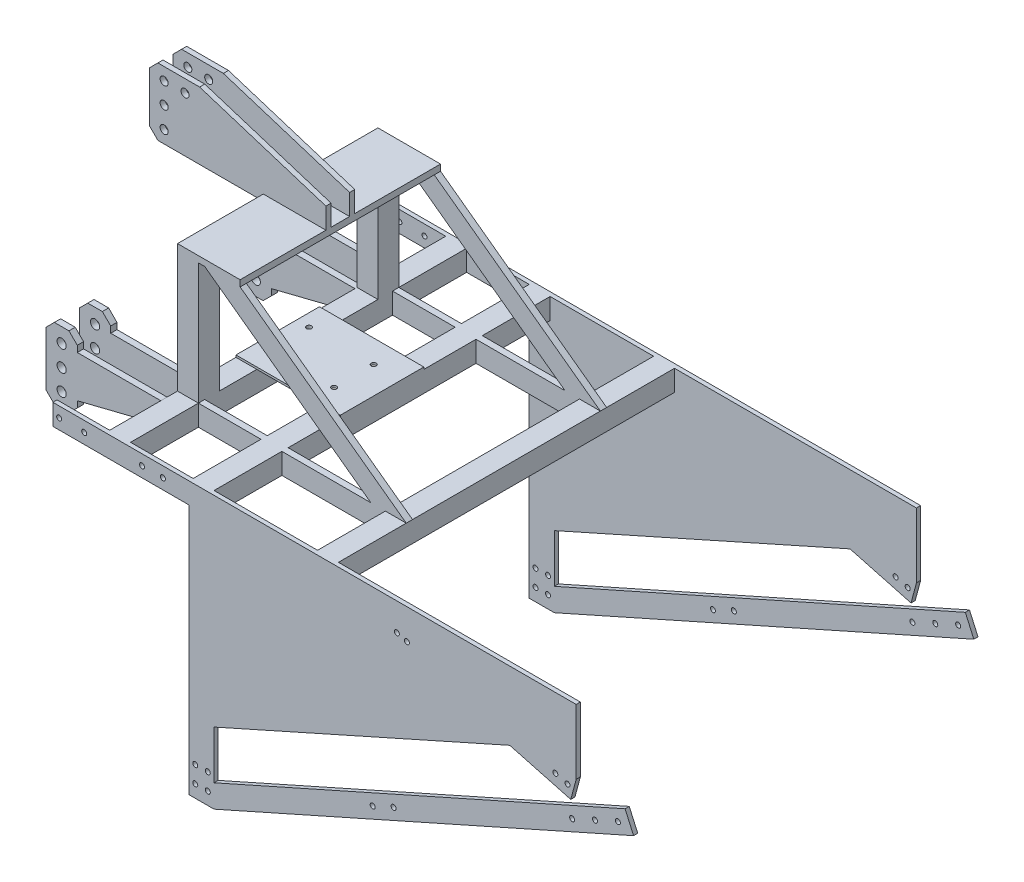
SolidWorks part; units mm, degrees
ref_plane "前视基准面" through (0, 0, 0) normal (0, 0, 1) x (1, 0, 0)
ref_plane "上视基准面" through (0, 0, 0) normal (0, 1, 0) x (1, 0, 0)
ref_plane "右视基准面" through (0, 0, 0) normal (1, 0, 0) x (0, 0, -1)
sketch "草图1" plane through (0, 0, 0) normal (0, 0, 1) x (1, 0, 0)
  line L1 (0, 0) -> (50, 0)
  line L2 (0, 0) -> (0, 50)
  line L3 (0, 50) -> (50, 50)
  line L4 (50, 0) -> (50, 50)
  line L5 (5, 5) -> (45, 5)
  line L6 (5, 5) -> (5, 45)
  line L7 (5, 45) -> (45, 45)
  line L8 (45, 5) -> (45, 45)
  dimension "D1" = 5
  dimension "D2" = 5
  dimension "D3" = 5
  dimension "D4" = 5
extrude "凸台-拉伸1" add sketch "草图1" along normal mid plane 805
sketch "草图2" plane through (0, 0, 402.5) normal (0, 0, 1) x (1, 0, 0)
  line L0 (-237.8943, -601) -> (767.0057, -153.5897)
  line L1 (50, 50) -> (-250, 50)
  line L2 (746.6689, -107.9124) -> (767.0057, -153.5897)
  line L3 (43.4174, 0) -> (-237.8943, 0)
  line L4 (629.5555, -105.2914) -> (616.6145, -153.5877)
  line L5 (-250, 50) -> (-297.8943, 50)
  line L6 (-237.8943, 0) -> (-237.8943, -546.2682)
  line L7 (-237.8943, -601) -> (-297.8943, -601)
  line L8 (-297.8943, 0) -> (-297.8943, -601)
  line L9 (-297.8943, 50) -> (-497.8943, 50)
  line L10 (50, 50) -> (629.5555, -105.2914)
  line L11 (43.4174, 0) -> (616.6145, -153.5877)
  line L12 (-497.8943, 50) -> (-577.8943, 50)
  line L13 (-497.8943, 0) -> (-297.8943, 0)
  line L15 (-577.8943, 0) -> (-497.8943, 0)
  line L16 (-385.3943, 150) -> (-385.3943, -14.3313) construction
  line L17 (-577.8943, 50) -> (-623.8943, 50)
  line L18 (-623.8943, 50) -> (-623.8943, 0)
  line L19 (746.6689, -107.9124) -> (-237.8943, -546.2682)
  line L20 (-623.8943, 0) -> (-577.8943, 0)
  circle A0 centre (-282.8943, -531) radius 6
  circle A1 centre (-252.8943, -531) radius 6
  circle A2 centre (-282.8943, -571) radius 6
  circle A3 centre (-252.8943, -571) radius 6
  circle A4 centre (142.1057, -404.4472) radius 6
  circle A5 centre (-267.8943, -248) radius 6
  circle A6 centre (-267.8943, -284) radius 6
  circle A7 centre (192.1057, -382.1858) radius 6
  circle A8 centre (729.4309, -142.9532) radius 6
  circle A9 centre (674.6182, -167.3574) radius 6
  circle A10 centre (619.8055, -191.7616) radius 6
  circle A11 centre (608.5961, -125.5573) radius 6
  circle A12 centre (579.6184, -117.7927) radius 6
  circle A13 centre (-608.8943, 25) radius 6
  circle A14 centre (-548.8943, 25) radius 6
  circle A15 centre (-360.3943, 25) radius 6
  circle A16 centre (-410.3943, 25) radius 6
  circle A17 centre (200, -16.0743) radius 6
  circle A18 centre (224.1481, -22.5448) radius 6
  dimension "D4" = 15
  dimension "D5" = 30
  dimension "D6" = 15
  dimension "D7" = 30
  dimension "D8" = 30
  dimension "D9" = 40
  dimension "D10" = 36
  dimension "D11" = 248
  dimension "D12" = 15
  dimension "D2" = 30
  dimension "D13" = 30
  dimension "D17" = 50
  dimension "D19" = 30
  dimension "D20" = 60
  dimension "D21" = 60
  dimension "D22" = 15
  dimension "D23" = 30
  dimension "D27" = 25
  dimension "D28" = 25
  dimension "D1" = 24
  dimension "D3" = 601
  dimension "D14" = 60
  dimension "D15" = 601
  dimension "D16" = 50
  dimension "D18" = 1100
  dimension "D25" = 200
extrude "凸台-拉伸2" add sketch "草图2" along normal blind 10
sketch "草图3" plane through (0, 0, 402.5) normal (0, 0, -1) x (-1, 0, 0)
  line L1 (297.8943, 50) -> (247.8943, 50)
  line L2 (297.8943, 50) -> (297.8943, 0)
  line L3 (297.8943, 0) -> (247.8943, 0)
  line L4 (247.8943, 50) -> (247.8943, 0)
  line L5 (252.8943, 5) -> (292.8943, 5)
  line L6 (252.8943, 5) -> (252.8943, 45)
  line L7 (252.8943, 45) -> (292.8943, 45)
  line L8 (292.8943, 5) -> (292.8943, 45)
  dimension "D1" = 40
  dimension "D2" = 5
  dimension "D3" = 5
extrude "凸台-拉伸3" add sketch "草图3" along normal up to surface (805 mm away) up to face at (25, 25, -402.5)
sketch "草图4" plane through (0, 0, -402.5) normal (0, 0, -1) x (-1, 0, 0)
  line L0 (-612.8098, -100.8044) -> (-50, 50)
  line L1 (-50, 50) -> (297.8943, 50)
  line L2 (297.8943, 0) -> (297.8943, -601)
  line L3 (297.8943, -601) -> (237.8943, -601)
  line L4 (237.8943, -601) -> (-767.0057, -153.5897)
  line L5 (297.8943, 0) -> (497.8943, 0)
  line L6 (-746.6689, -107.9124) -> (237.8943, -546.2682)
  line L7 (237.8943, -546.2682) -> (237.8943, 0)
  line L8 (237.8943, 0) -> (-43.4174, 0)
  line L9 (-767.0057, -153.5897) -> (-746.6689, -107.9124)
  line L10 (497.8943, 50) -> (577.8943, 50)
  line L11 (-43.4174, 0) -> (-616.6145, -153.5877)
  line L12 (-616.6145, -153.5877) -> (-629.5555, -105.2914)
  line L13 (-629.5555, -105.2914) -> (-612.8098, -100.8044)
  line L14 (497.8943, 50) -> (297.8943, 50)
  line L15 (-50, 50) -> (623.8943, 50) construction
  line L17 (577.8943, 0) -> (497.8943, 0)
  line L18 (577.8943, 50) -> (623.8943, 50)
  line L19 (623.8943, 50) -> (623.8943, 0)
  line L20 (623.8943, 50) -> (623.8943, 0) construction
  line L21 (623.8943, 0) -> (577.8943, 0)
  circle A0 centre (267.8943, -248) radius 6
  circle A1 centre (267.8943, -284) radius 6
  circle A2 centre (252.8943, -531) radius 6
  circle A3 centre (282.8943, -531) radius 6
  circle A4 centre (282.8943, -571) radius 6
  circle A5 centre (252.8943, -571) radius 6
  circle A6 centre (-192.1057, -382.1858) radius 6
  circle A7 centre (-142.1057, -404.4472) radius 6
  circle A8 centre (-608.5961, -125.5573) radius 6
  circle A9 centre (-579.6184, -117.7927) radius 6
  circle A10 centre (-674.6182, -167.3574) radius 6
  circle A11 centre (-729.4309, -142.9532) radius 6
  circle A12 centre (-619.8055, -191.7616) radius 6
  circle A13 centre (608.8943, 25) radius 6
  circle A14 centre (548.8943, 25) radius 6
extrude "凸台-拉伸4" add sketch "草图4" along normal blind 10
ref_plane "基准面1" through (0, 0, 232.5) normal (0, 0, 1) x (1, 0, 0)
ref_plane "基准面2" through (0, 0, -232.5) normal (0, 0, 1) x (1, 0, 0)
sketch "草图5" plane through (0, 0, 232.5) normal (0, 0, 1) x (1, 0, 0)
  line L0 (-497.8943, 50) -> (-497.8943, 0)
  line L1 (-497.8943, 50) -> (-697.8943, 50)
  line L2 (-697.8943, 50) -> (-697.8943, 65)
  line L3 (-717.8943, 85) -> (-752.8943, 85)
  line L4 (-772.8943, 65) -> (-772.8943, -65)
  line L5 (-752.8943, -85) -> (-717.8943, -85)
  line L6 (-752.8943, 85) -> (-772.8943, 65)
  line L7 (-297.8943, 0) -> (-297.8943, -601) construction
  line L8 (-697.8943, -65) -> (-697.8943, -50)
  line L9 (-697.8943, 65) -> (-717.8943, 85)
  line L10 (-697.8943, -50) -> (-497.8943, 0)
  line L11 (-717.8943, -85) -> (-697.8943, -65)
  line L12 (-772.8943, -65) -> (-752.8943, -85)
  circle A2 centre (-735.3943, 50) radius 11
  circle A3 centre (-735.3943, 0) radius 11
  circle A5 centre (-735.3943, -50) radius 11
  point P0 (-772.8943, -85)
  point P1 (-697.8943, 85)
  point P6 (-772.8943, 85)
  point P12 (-697.8943, -85)
  dimension "D7" = 50
  dimension "D2" = 35
  dimension "D4" = 75
  dimension "D6" = 35
  dimension "D9" = 200
extrude "凸台-拉伸5" add sketch "草图5" along normal mid plane 95
sketch "草图7" plane through (0, 0, -232.5) normal (0, 0, 1) x (1, 0, 0)
  line L0 (-772.8943, 65) -> (-772.8943, -65)
  line L1 (-752.8943, -85) -> (-717.8943, -85)
  line L2 (-697.8943, -65) -> (-697.8943, -50)
  line L4 (-497.8943, 0) -> (-497.8943, 50)
  line L5 (-497.8943, 50) -> (-697.8943, 50)
  line L6 (-697.8943, 50) -> (-697.8943, 65)
  line L7 (-717.8943, 85) -> (-752.8943, 85)
  line L8 (-697.8943, 65) -> (-717.8943, 85)
  line L9 (-752.8943, 85) -> (-772.8943, 65)
  line L10 (-772.8943, -65) -> (-752.8943, -85)
  line L11 (-697.8943, -50) -> (-497.8943, 0)
  line L12 (-717.8943, -85) -> (-697.8943, -65)
  circle A2 centre (-735.3943, 50) radius 11
  circle A3 centre (-735.3943, 0) radius 11
  circle A5 centre (-735.3943, -50) radius 11
  point P0 (-772.8943, 85)
  point P1 (-772.8943, -85)
  point P3 (-697.8943, -85)
  point P12 (-697.8943, 85)
  point P22 (-772.8943, 85)
  dimension "D1" = 50
extrude "凸台-拉伸6" add sketch "草图7" along normal mid plane 95 separate body
sketch "草图10" plane through (0, 85, 0) normal (0, 1, 0) x (1, 0, 0)
  line L0 (-497.8943, 280) -> (-697.8943, 280) construction
  line L1 (-804.976, 265) -> (-454.4331, 265)
  line L2 (-804.976, 265) -> (-804.976, 200)
  line L3 (-804.976, 200) -> (-454.4331, 200)
  line L4 (-454.4331, 265) -> (-454.4331, 200)
  dimension "D1" = 65
  dimension "D2" = 15
extrude "切除-拉伸6" cut sketch "草图10" against normal through all
sketch "草图11" plane through (0, 0, -402.5) normal (0, 0, 1) x (1, 0, 0)
  line L1 (-497.8943, 50) -> (-447.8943, 50)
  line L2 (-497.8943, 50) -> (-497.8943, 0)
  line L3 (-497.8943, 0) -> (-447.8943, 0)
  line L4 (-447.8943, 50) -> (-447.8943, 0)
  line L5 (-492.8943, 45.3872) -> (-452.8943, 45.3872)
  line L6 (-492.8943, 45.3872) -> (-492.8943, 5.3872)
  line L7 (-492.8943, 5.3872) -> (-452.8943, 5.3872)
  line L8 (-452.8943, 45.3872) -> (-452.8943, 5.3872)
  dimension "D1" = 40
  dimension "D2" = 50
  dimension "D3" = 5
extrude "凸台-拉伸7" add sketch "草图11" along normal up to surface (805 mm away) up to face at (198.1057, -382.1858, 402.5)
sketch "草图12" plane through (0, 85, 0) normal (0, 1, 0) x (1, 0, 0)
  line L0 (-497.8943, -402.5) -> (-497.8943, 185) construction
  line L1 (-813.5215, -200) -> (-497.8943, -200)
  line L2 (-813.5215, -200) -> (-813.5215, -265)
  line L3 (-813.5215, -265) -> (-497.8943, -265)
  line L4 (-497.8943, -200) -> (-497.8943, -265)
  line L6 (-497.8943, -280) -> (-697.8943, -280) construction
  dimension "D1" = 65
  dimension "D2" = 15
extrude "切除-拉伸7" cut sketch "草图12" against normal through all
sketch "草图13" plane through (0, 0, 232.5) normal (0, 0, 1) x (1, 0, 0)
  line L1 (-447.8943, 50) -> (0, 50)
  line L2 (-447.8943, 50) -> (-447.8943, 0)
  line L3 (-447.8943, 0) -> (0, 0)
  line L4 (0, 50) -> (0, 0)
extrude "凸台-拉伸8" add sketch "草图13" along normal mid plane 15
sketch "草图14" plane through (0, 0, -232.5) normal (0, 0, 1) x (1, 0, 0)
  line L1 (-447.8943, 50) -> (0, 50)
  line L2 (-447.8943, 50) -> (-447.8943, 0)
  line L3 (-447.8943, 0) -> (0, 0)
  line L4 (0, 50) -> (0, 0)
extrude "凸台-拉伸9" add sketch "草图14" along normal mid plane 15
sketch "草图15" plane through (0, 0, 0) normal (0, 0, 1) x (1, 0, 0)
  line L0 (-670.3943, 341) -> (-297.8943, 341)
  line L1 (-770.3943, 481.7) -> (-750.3943, 501.7)
  line L3 (-770.3943, 361) -> (-750.3943, 341)
  line L6 (-297.8943, 341) -> (-297.8943, 404.9245)
  line L7 (-750.3943, 501.7) -> (-645.3943, 501.7)
  line L8 (-297.8943, 404.9245) -> (-645.3943, 501.7)
  line L9 (-770.3943, 371) -> (-770.3943, 361)
  line L10 (-750.3943, 341) -> (-670.3943, 341)
  line L11 (-770.3943, 371) -> (-770.3943, 481.7)
  circle A0 centre (-735.3943, 471.7) radius 9.65
  circle A3 centre (-735.3943, 371) radius 9.65
  circle A4 centre (-735.3943, 421.7) radius 9.65
  circle A6 centre (-685.3943, 471.7) radius 9.65
  point P20 (-770.3943, 341)
  dimension "D1" = 19.3
  dimension "D2" = 50
  dimension "D5" = 50
extrude "凸台-拉伸10" add sketch "草图15" along normal mid plane 69 separate body
sketch "草图16" plane through (0, 501.7, 0) normal (0, 1, 0) x (1, 0, 0)
  line L0 (-645.3943, 34.5) -> (-750.3943, 34.5) construction
  line L1 (-821.6581, 22.25) -> (-221.0953, 22.25)
  line L2 (-821.6581, 22.25) -> (-821.6581, -22.25)
  line L3 (-821.6581, -22.25) -> (-221.0953, -22.25)
  line L4 (-221.0953, 22.25) -> (-221.0953, -22.25)
  dimension "D1" = 44.5
  dimension "D2" = 600.5628
  dimension "D3" = 12.25
extrude "切除-拉伸8" cut sketch "草图16" against normal blind 200
sketch "草图19" plane through (-497.8943, 0, 0) normal (-1, 0, 0) x (0, 0, 1)
  line L0 (-240, 341) -> (-240, 356)
  line L1 (-240, 356) -> (240, 356)
  line L2 (-240, 341) -> (240, 341)
  line L3 (240, 356) -> (240, 341)
extrude "凸台-拉伸11" add sketch "草图19" against normal blind 200
sketch "草图20" plane through (0, 0, 240) normal (0, 0, 1) x (1, 0, 0)
  line L0 (-347.8943, 341) -> (50, 50)
  line L5 (-34.6995, 50) -> (-432.5938, 341)
  line L6 (-347.8943, 341) -> (-432.5938, 341)
  line L7 (50, 50) -> (-34.6995, 50)
  line L9 (-297.8943, 341) -> (-497.8943, 341) construction
  line L12 (50, 50) -> (-623.8943, 50) construction
extrude "凸台-拉伸12" add sketch "草图20" against normal blind 15
sketch "草图21" plane through (0, 0, -225) normal (0, 0, 1) x (1, 0, 0)
  line L0 (50, 50) -> (-347.8943, 341)
  line L1 (-347.8943, 341) -> (-432.5938, 341)
  line L2 (-432.5938, 341) -> (-34.6995, 50)
  line L3 (-34.6995, 50) -> (50, 50)
extrude "凸台-拉伸13" add sketch "草图21" against normal blind 15
sketch "草图23" plane through (0, 50, 0) normal (0, 1, 0) x (1, 0, 0)
  line L1 (-497.8943, -240) -> (-447.8943, -240)
  line L2 (-497.8943, -240) -> (-497.8943, -190)
  line L3 (-497.8943, -190) -> (-447.8943, -190)
  line L4 (-447.8943, -240) -> (-447.8943, -190)
  line L5 (-492.8943, -235) -> (-452.8943, -235)
  line L6 (-492.8943, -235) -> (-492.8943, -195)
  line L7 (-492.8943, -195) -> (-452.8943, -195)
  line L8 (-452.8943, -235) -> (-452.8943, -195)
  line L9 (-497.8943, 240) -> (-447.8943, 240)
  line L10 (-497.8943, 240) -> (-497.8943, 190)
  line L11 (-497.8943, 190) -> (-447.8943, 190)
  line L12 (-447.8943, 240) -> (-447.8943, 190)
  line L13 (-492.8943, 235) -> (-452.8943, 235)
  line L14 (-492.8943, 235) -> (-492.8943, 195)
  line L15 (-492.8943, 195) -> (-452.8943, 195)
  line L16 (-452.8943, 235) -> (-452.8943, 195)
  dimension "D1" = 5
  dimension "D2" = 5
  dimension "D3" = 5
extrude "凸台-拉伸14" add sketch "草图23" along normal up to surface (291 mm away) up to face at (-482.4517, 341, -0.75)
sketch "草图24" plane through (0, 0, 240) normal (0, 0, 1) x (1, 0, 0)
  line L0 (-347.8943, 341) -> (-347.8943, 356)
  line L1 (-297.8943, 356) -> (-497.8943, 356) construction
  line L2 (-347.8943, 356) -> (-347.8943, 406)
  line L5 (-645.3943, 501.7) -> (-750.3943, 501.7) construction
  line L6 (-650.3943, 501.7) -> (-347.8943, 406)
  line L7 (-347.8943, 341) -> (-259.9702, 341)
  line L8 (-259.9702, 341) -> (-259.9702, 501.7)
  line L9 (-259.9702, 501.7) -> (-259.9702, 527.4368)
  line L10 (-259.9702, 527.4368) -> (-650.3943, 527.4368)
  line L11 (-650.3943, 527.4368) -> (-650.3943, 501.7)
extrude "切除-拉伸9" cut sketch "草图24" against normal through all
sketch "草图25" plane through (0, 50, 0) normal (0, 1, 0) x (1, 0, 0)
  line L0 (-447.8943, -190) -> (-447.8943, 190) construction
  line L1 (-447.8943, 100) -> (-247.8943, 100)
  line L2 (-297.8943, 225) -> (-297.8943, -225) construction
  line L3 (-454.6865, -100) -> (-247.8943, -100)
  line L4 (-247.8943, 100) -> (-247.8943, -100)
  line L5 (-247.8943, 225) -> (-247.8943, -225) construction
  line L6 (-497.8943, 0) -> (61.9576, 0) construction
  line L7 (-497.8943, -22.25) -> (-497.8943, 22.25) construction
  line L8 (-447.8943, 100) -> (-497.8943, 100)
  line L9 (-497.8943, 34.5) -> (-497.8943, 240) construction
  line L10 (-497.8943, 100) -> (-497.8943, -100)
  line L11 (-497.8943, -240) -> (-497.8943, -34.5) construction
  line L12 (-497.8943, -100) -> (-454.6865, -100)
  circle A0 centre (-467.8943, 45) radius 6
  circle A1 centre (-312.8943, 45) radius 6
  circle A2 centre (-312.8943, -50) radius 6
  circle A3 centre (-467.8943, -50) radius 6
  dimension "D3" = 15
  dimension "D4" = 95
  dimension "D5" = 155
  dimension "D6" = 155
  dimension "D7" = 95
  dimension "D8" = 50
  dimension "D9" = 50
  dimension "D10" = 15
  dimension "D1" = 200
  dimension "D2" = 100
extrude "凸台-拉伸15" add sketch "草图25" along normal blind 5
sketch "草图26" plane through (0, 55, 0) normal (0, 1, 0) x (1, 0, 0)
  circle A0 centre (-467.8943, -50) radius 6
  circle A1 centre (-467.8943, 45) radius 6
extrude "切除-拉伸10" cut sketch "草图26" against normal through all
sketch "草图27" plane through (0, 0, 412.5) normal (0, 0, 1) x (1, 0, 0)
  circle A0 centre (-267.8943, -248) radius 6
extrude "凸台-拉伸16" add sketch "草图27" against normal up to vertex
sketch "草图29" plane through (0, 0, 412.5) normal (0, 0, 1) x (1, 0, 0)
  circle A0 centre (-267.8943, -284) radius 6
extrude "凸台-拉伸17" add sketch "草图29" against normal blind 10
sketch "草图30" plane through (0, 0, -412.5) normal (0, 0, -1) x (-1, 0, 0)
  circle A0 centre (267.8943, -248) radius 6
extrude "凸台-拉伸18" add sketch "草图30" against normal blind 10
sketch "草图31" plane through (0, 0, -412.5) normal (0, 0, -1) x (-1, 0, 0)
  circle A0 centre (267.8943, -284) radius 6
extrude "凸台-拉伸19" add sketch "草图31" against normal blind 10
sketch "草图32" plane through (0, 0, 412.5) normal (0, 0, 1) x (1, 0, 0)
  line L0 (-237.8943, 0) -> (-237.8943, -400.6751)
  line L1 (-237.8943, -546.2682) -> (-237.8943, 0) construction
  line L2 (-237.8943, -400.6751) -> (429.6142, -103.4811)
  line L3 (43.4174, 0) -> (616.6145, -153.5877) construction
  line L4 (429.6142, -103.4811) -> (43.4174, 0)
  line L5 (43.4174, 0) -> (-237.8943, 0)
extrude "凸台-拉伸21" add sketch "草图32" against normal blind 10 contours L5 L0 L2 L4
sketch "草图33" plane through (0, 0, -412.5) normal (0, 0, -1) x (-1, 0, 0)
  line L0 (237.8943, 0) -> (237.8943, -400.6751)
  line L1 (237.8943, -400.6751) -> (-429.6142, -103.4811)
  line L2 (-429.6142, -103.4811) -> (-50, 0)
  line L3 (-50, 0) -> (237.8943, 0)
extrude "凸台-拉伸23" add sketch "草图33" against normal blind 10 contours L3 L0 L1 L2
sketch "草图34" plane through (0, 0, 412.5) normal (0, 0, 1) x (1, 0, 0)
  line L0 (50, 50) -> (629.5555, -105.2914)
  line L1 (629.5555, -105.2914) -> (629.5555, 50)
  line L2 (629.5555, 50) -> (50, 50)
extrude "凸台-拉伸26" add sketch "草图34" against normal blind 10
sketch "草图35" plane through (0, 0, -412.5) normal (0, 0, -1) x (-1, 0, 0)
  line L0 (-629.5555, -105.2914) -> (-629.5555, 50)
  line L1 (-629.5555, 50) -> (-50, 50)
  line L2 (-50, 50) -> (-629.5555, -105.2914)
extrude "凸台-拉伸28" add sketch "草图35" against normal blind 10
sketch "草图36" plane through (0, 0, 412.5) normal (0, 0, 1) x (1, 0, 0)
  line L0 (-237.8943, -400.6751) -> (-237.8943, -430.6751)
  line L1 (-237.8943, -546.2682) -> (-237.8943, -400.6751) construction
  line L2 (-237.8943, -430.6751) -> (470.4607, -114.4259)
  line L3 (429.6142, -103.4811) -> (616.6145, -153.5877) construction
  line L4 (470.4607, -114.4259) -> (429.6142, -103.4811)
  line L5 (429.6142, -103.4811) -> (-237.8943, -400.6751)
extrude "凸台-拉伸29" add sketch "草图36" against normal blind 10
sketch "草图37" plane through (0, 0, -412.5) normal (0, 0, -1) x (-1, 0, 0)
  line L0 (237.8943, -400.6751) -> (237.8943, -430.6751)
  line L1 (237.8943, -400.6751) -> (237.8943, -546.2682) construction
  line L2 (237.8943, -430.6751) -> (-470.4607, -114.4259)
  line L3 (-470.4607, -114.4259) -> (-429.6142, -103.4811)
  line L4 (-616.6145, -153.5877) -> (-429.6142, -103.4811) construction
  line L5 (-429.6142, -103.4811) -> (237.8943, -400.6751)
extrude "凸台-拉伸30" add sketch "草图37" against normal blind 10
